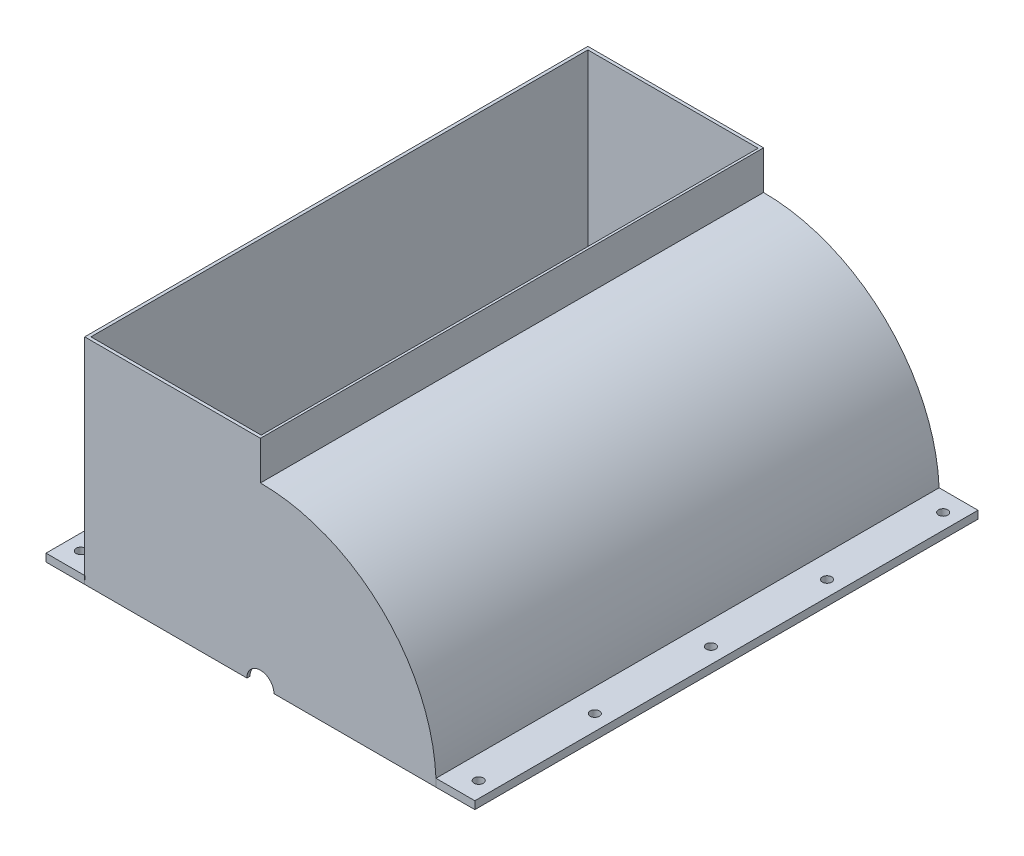
from build123d import *

# Parameters (mm, degrees)
SKETCH1_W               = 50
SKETCH1_H               = 10
BOSS_EXTRUDE1_DEPTH     = 325
BOSS_EXTRUDE4_DEPTH     = 4
BOSS_EXTRUDE5_START     = -4
BOSS_EXTRUDE5_DEPTH     = 4
SKETCH6_R               = 6
CUT_EXTRUDE1_DEPTH      = 570.634093081
LPATTERN1_COUNT         = 3
LPATTERN1_PITCH         = 150
LPATTERN2_COUNT         = 3
LPATTERN2_PITCH         = 150
CUT_EXTRUDE2_DEPTH      = 801.848300242
CUT_EXTRUDE2_DEPTH_BACK = 801.848300242
SKETCH7_R               = 17.5
SKETCH8_W               = 720.760198568
SKETCH8_H               = 761.43709551
CUT_EXTRUDE3_DEPTH      = 100


with BuildPart() as part:
    # Sketch1 → Boss-Extrude1 (new, symmetric)
    with BuildSketch(Plane.XY):
        with Locations((-252, 5)):
            Rectangle(SKETCH1_W, SKETCH1_H)
        with BuildLine():
            ThreePointArc((-226.779628715, 10), (-226.944900492, 5.00121394), (-227, 0))
            Line((-227, 0), (-226.920690991, 0))
            Line((-226.920690991, 0), (-223, 0))
            Line((-223, 0), (-223, 10))
            Line((-223, 10), (-226.779628715, 10))
        make_face()
        with BuildLine():
            ThreePointArc((-223, 42.426406871), (-225.473494157, 26.281237274), (-226.779628715, 10))
            Line((-226.779628715, 10), (-223, 10))
            Line((-223, 10), (-223, 42.426406871))
        make_face()
        with BuildLine():
            Line((-227, 377), (-227, 10))
            Line((-227, 10), (-226.779628715, 10))
            ThreePointArc((-226.779628715, 10), (-225.473494157, 26.281237274), (-223, 42.426406871))
            Line((-223, 42.426406871), (-223, 377))
            Line((-223, 377), (-227, 377))
        make_face()
        with BuildLine():
            Line((-3, 377), (-3, 226.980175346))
            ThreePointArc((-3, 226.980175346), (-1.500032751, 226.995043782), (0, 227))
            Line((0, 227), (0, 377))
            Line((0, 377), (-3, 377))
        make_face()
        with BuildLine():
            Line((-3, 226.980175346), (-3, 222.979819715))
            ThreePointArc((-3, 222.979819715), (-1.500033937, 222.994954872), (0, 223))
            Line((0, 223), (0, 227))
            ThreePointArc((0, 227), (-1.500032751, 226.995043782), (-3, 226.980175346))
        make_face()
        with BuildLine():
            ThreePointArc((0, 223), (157.684812205, 157.684812205), (223, 0))
            Line((223, 0), (226.779628715, 0))
            Line((226.779628715, 0), (226.779628715, 10))
            ThreePointArc((226.779628715, 10), (156.937885802, 164.010670385), (0, 227))
            Line((0, 227), (0, 223))
        make_face()
        with BuildLine():
            Line((277, 10), (226.779628715, 10))
            ThreePointArc((226.779628715, 10), (226.944900492, 5.00121394), (227, 0))
            Line((227, 0), (277, 0))
            Line((277, 0), (277, 10))
        make_face()
    extrude(amount=BOSS_EXTRUDE1_DEPTH, both=True)

    # Sketch3 → Boss-Extrude4 (add)
    with BuildSketch(Plane.XY.offset(325)):
        with BuildLine():
            Line((-223, 0), (223, 0))
            ThreePointArc((223, 0), (156.620560592, 158.741928929), (-3, 222.979819715))
            Line((-3, 222.979819715), (-3, 377))
            Line((-3, 377), (-223, 377))
            Line((-223, 377), (-223, 0))
        make_face()
    extrude(amount=-BOSS_EXTRUDE4_DEPTH)

    # Sketch4 → Boss-Extrude5 (add)
    with BuildSketch(Plane(origin=(0, 0, -325), x_dir=(-1, 0, 0), z_dir=(0, 0, -1)).offset(BOSS_EXTRUDE5_START)):
        with BuildLine():
            Line((-223, 0), (223, 0))
            Line((223, 0), (223, 377))
            Line((223, 377), (3, 377))
            Line((3, 377), (3, 222.979819715))
            ThreePointArc((3, 222.979819715), (-156.620560592, 158.741928929), (-223, 0))
        make_face()
    extrude(amount=BOSS_EXTRUDE5_DEPTH)

    # Sketch6 → Cut-Extrude1 (cut, symmetric)
    with BuildSketch(Plane.XZ):
        with Locations((257, 0)):
            Circle(SKETCH6_R)
        with Locations(Location((-257, 0, 0), (0, 0, 90))):
            Circle(SKETCH6_R)
    cut_extrude1 = extrude(amount=CUT_EXTRUDE1_DEPTH, both=True, mode=Mode.SUBTRACT)

    # LPattern1: Cut-Extrude1 ×3
    with Locations(*[(0, 0, -i * LPATTERN1_PITCH) for i in range(1, LPATTERN1_COUNT)]):
        add(cut_extrude1, mode=Mode.SUBTRACT)

    # LPattern2: Cut-Extrude1 ×3
    with Locations(*[(0, 0, i * LPATTERN2_PITCH) for i in range(1, LPATTERN2_COUNT)]):
        add(cut_extrude1, mode=Mode.SUBTRACT)

    # Sketch7 → Cut-Extrude2 (cut, two sides: drawn at the far end of the back side and taken through both)
    with BuildSketch(Plane.XY.offset(325).offset(-CUT_EXTRUDE2_DEPTH_BACK)):
        Circle(SKETCH7_R)
    extrude(amount=CUT_EXTRUDE2_DEPTH + CUT_EXTRUDE2_DEPTH_BACK, mode=Mode.SUBTRACT)

    # Sketch8 → Cut-Extrude3 (cut)
    with BuildSketch(Plane(origin=(0, 377, 0), x_dir=(1, 0, 0), z_dir=(0, 1, 0))):
        with Locations((4.182407147, 0)):
            Rectangle(SKETCH8_W, SKETCH8_H)
    extrude(amount=-CUT_EXTRUDE3_DEPTH, mode=Mode.SUBTRACT)


solid = part.part
